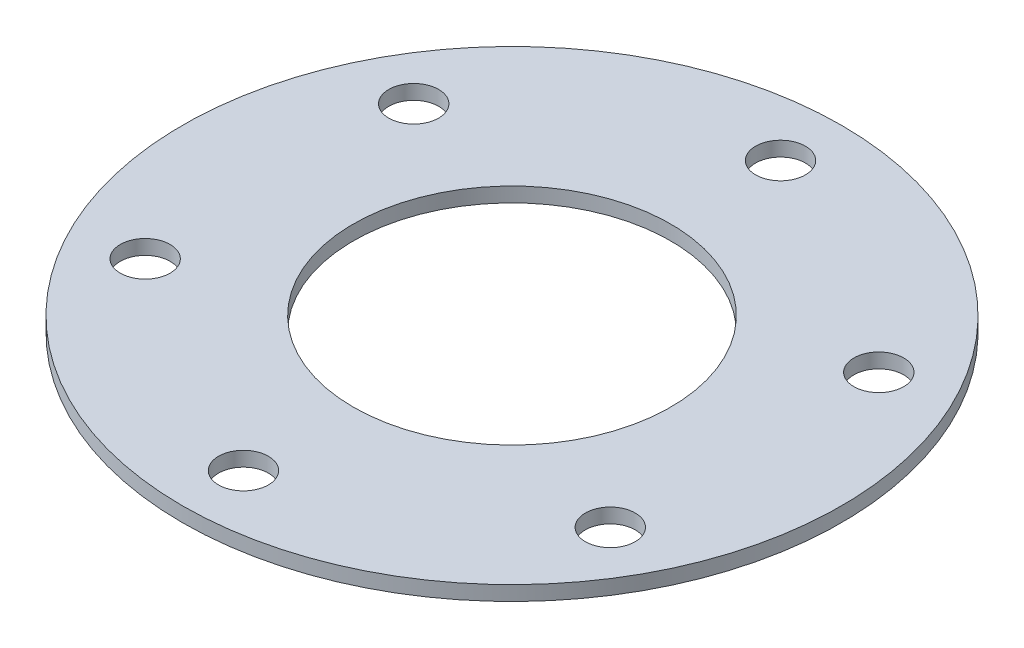
from build123d import *

# Parameters (mm, degrees)
SKETCH_1_R              = 67.5
SKETCH_1_R_2            = 32.5
EXTRUDE_1_DEPTH         = 3
HOLE_WIZARD_M12_1_D     = 10.2
HOLE_WIZARD_M12_1_DEPTH = 5
HOLE_WIZARD_M12_1_TIP   = 3.064389157


with BuildPart() as part:
    # 草图1 → 凸台-拉伸1 (new body)
    with BuildSketch(Plane(origin=(0, 0, 0), x_dir=(1, 0, 0), z_dir=(0, 1, 0))):
        with Locations(Location((0, 0, 0), (0, 0, 270))):
            Circle(SKETCH_1_R)
        with Locations(Location((0, 0, 0), (0, 0, 270))):
            Circle(SKETCH_1_R_2, mode=Mode.SUBTRACT)
    extrude(amount=EXTRUDE_1_DEPTH)

    # M12 螺纹孔的螺纹孔钻头1
    with Locations(Plane(origin=(0, 3, 0), x_dir=(1, 0, 0), z_dir=(0, 1, 0))):
        with Locations((0, 55), (-47.631397208, 27.5), (-47.631397208, -27.5), (0, -55), (47.631397208, -27.5), (47.631397208, 27.5)):
            Hole(HOLE_WIZARD_M12_1_D / 2, depth=HOLE_WIZARD_M12_1_DEPTH)
            with Locations((0, 0, -(HOLE_WIZARD_M12_1_DEPTH + HOLE_WIZARD_M12_1_TIP / 2))):  # 118° drill point
                Cone(0, HOLE_WIZARD_M12_1_D / 2, HOLE_WIZARD_M12_1_TIP, mode=Mode.SUBTRACT)


solid = part.part
